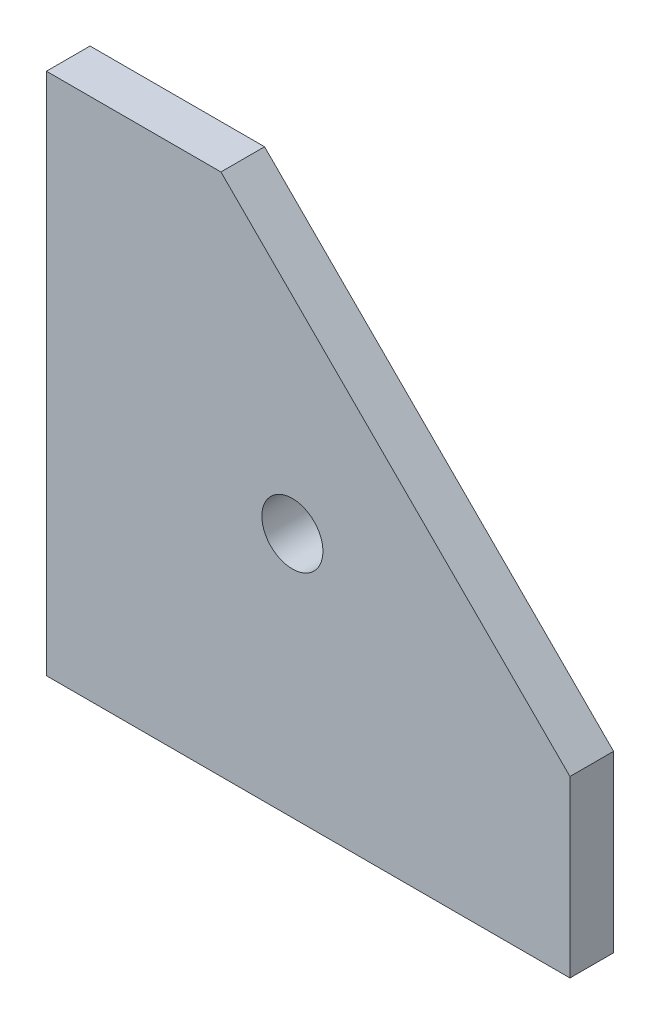
SolidWorks part; units mm, degrees
ref_plane "前视基准面" through (0, 0, 0) normal (0, 0, 1) x (1, 0, 0)
ref_plane "上视基准面" through (0, 0, 0) normal (0, 1, 0) x (1, 0, 0)
ref_plane "右视基准面" through (0, 0, 0) normal (1, 0, 0) x (0, 0, -1)
sketch "草图1" plane through (0, 0, 0) normal (0, 0, 1) x (1, 0, 0)
  line L0 (0, 120) -> (0, 0)
  line L1 (0, 0) -> (120, 0)
  line L2 (120, 0) -> (120, 40)
  line L3 (120, 40) -> (40, 120)
  line L4 (40, 120) -> (0, 120)
  dimension "D1" = 120
  dimension "D2" = 40
extrude "凸台-拉伸1" add sketch "草图1" along normal blind 10
hole_wizard "M16 螺纹孔1" positions "草图2" profile "草图3" tap size "M16" standard "GB" end condition through all
sketch "草图2" plane through (0, 0, 0) normal (0, 0, -1) x (-1, 0, 0)
  line L0 (0, 0) -> (-56.3804, 56.3804) construction
  line L2 (0, 0) -> (-120, 0) construction
  point P0 (-56.3804, 56.3804)
  dimension "D1" = 45
sketch "草图3" plane through (56.3804, 56.3804, 0) normal (1, 0, 0) x (0, 1, 0)
  line L0 (0, 0) -> (0, 10)
  line L1 (0, 10) -> (7, 10)
  line L2 (7, 10) -> (7, 0)
  line L5 (7, 0) -> (0, 0)
  line L11 (0, -6.35) -> (0, 107.95) construction
  dimension "通孔螺纹孔钻头直径" = 14
  dimension "通孔螺纹孔钻头深度" = 10
cosmetic thread "孔螺蚊线1" parameters "D2"=16
